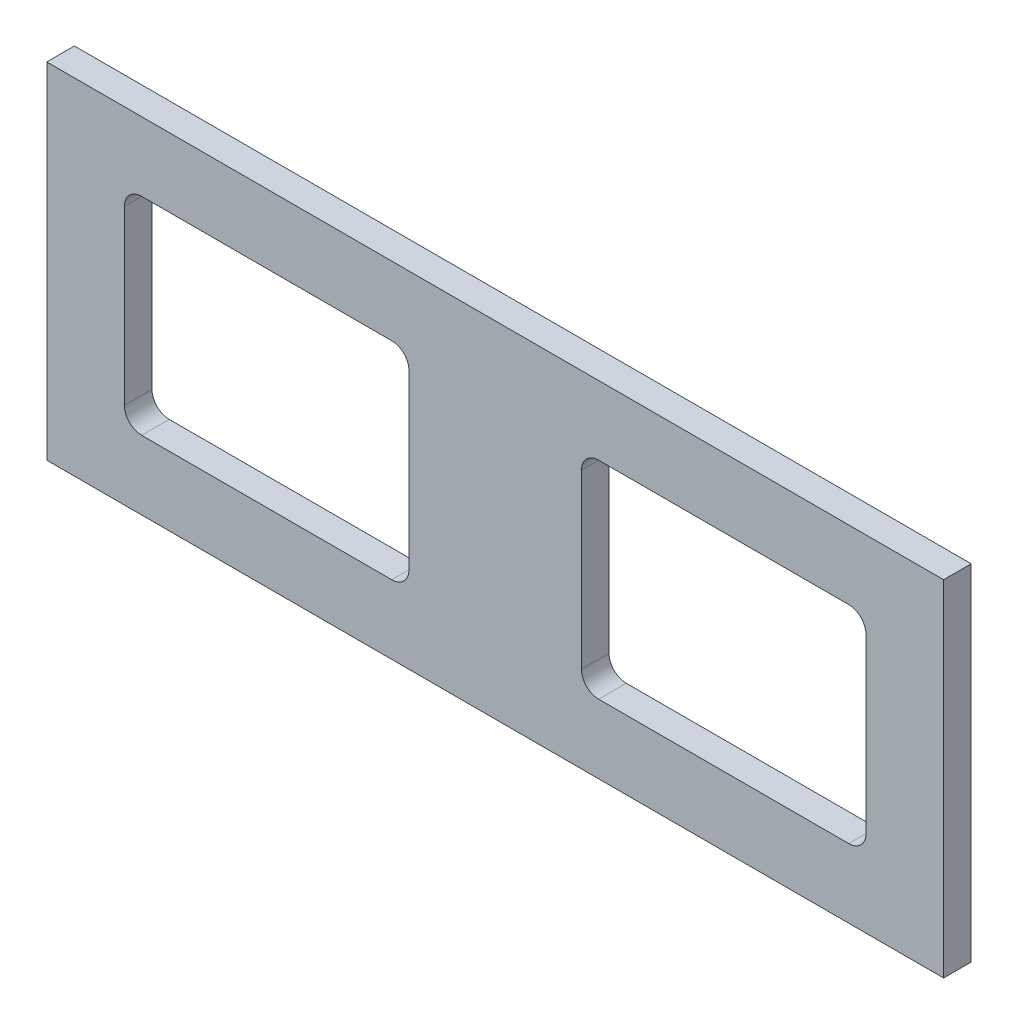
SolidWorks part; units mm, degrees
ref_plane "Front Plane" through (0, 0, 0) normal (0, 0, 1) x (1, 0, 0)
ref_plane "Top Plane" through (0, 0, 0) normal (0, 1, 0) x (1, 0, 0)
ref_plane "Right Plane" through (0, 0, 0) normal (1, 0, 0) x (0, 0, -1)
sketch "Sketch1" plane through (0, 0, 0) normal (0, 0, 1) x (1, 0, 0)
  line L0 (414.8492, -30.0349) -> (-105.1508, -30.0349)
  line L1 (154.8492, -123.1743) -> (154.8492, 384.2819) construction
  line L2 (-105.1508, -30.0349) -> (-105.1508, 169.9651)
  line L3 (-105.1508, 169.9651) -> (414.8492, 169.9651)
  line L4 (414.8492, 169.9651) -> (414.8492, -30.0349)
  line L5 (345.3501, 9.9651) -> (214.8492, 9.9651)
  line L6 (359.8492, 9.9651) -> (345.3501, 9.9651)
  line L7 (104.8492, 19.9651) -> (104.8492, 119.9651)
  line L8 (94.8492, 129.9651) -> (-50.1508, 129.9651)
  line L10 (-35.6516, 9.9651) -> (94.8492, 9.9651)
  line L11 (-60.1508, 119.9651) -> (-60.1508, 19.9651)
  line L12 (-50.1508, 9.9651) -> (-35.6516, 9.9651)
  line L13 (369.8492, 119.9651) -> (369.8492, 19.9651)
  line L14 (214.8492, 129.9651) -> (359.8492, 129.9651)
  line L15 (204.8492, 19.9651) -> (204.8492, 119.9651)
  arc A0 (-60.1508, 119.9651) -> (-50.1508, 129.9651) centre (-50.1508, 119.9651) cw
  arc A1 (-50.1508, 9.9651) -> (-60.1508, 19.9651) centre (-50.1508, 19.9651) cw
  arc A2 (94.8492, 9.9651) -> (104.8492, 19.9651) centre (94.8492, 19.9651) ccw
  arc A3 (94.8492, 129.9651) -> (104.8492, 119.9651) centre (94.8492, 119.9651) cw
  arc A4 (359.8492, 9.9651) -> (369.8492, 19.9651) centre (359.8492, 19.9651) ccw
  arc A5 (369.8492, 119.9651) -> (359.8492, 129.9651) centre (359.8492, 119.9651) ccw
  arc A6 (214.8492, 9.9651) -> (204.8492, 19.9651) centre (214.8492, 19.9651) cw
  arc A7 (214.8492, 129.9651) -> (204.8492, 119.9651) centre (214.8492, 119.9651) ccw
  point P3 (154.8492, -30.0349)
  dimension "D1" = 10
  dimension "D2" = 10
  dimension "D3" = 10
  dimension "D4" = 10
extrude "Boss-Extrude1" add sketch "Sketch1" along normal blind 16
